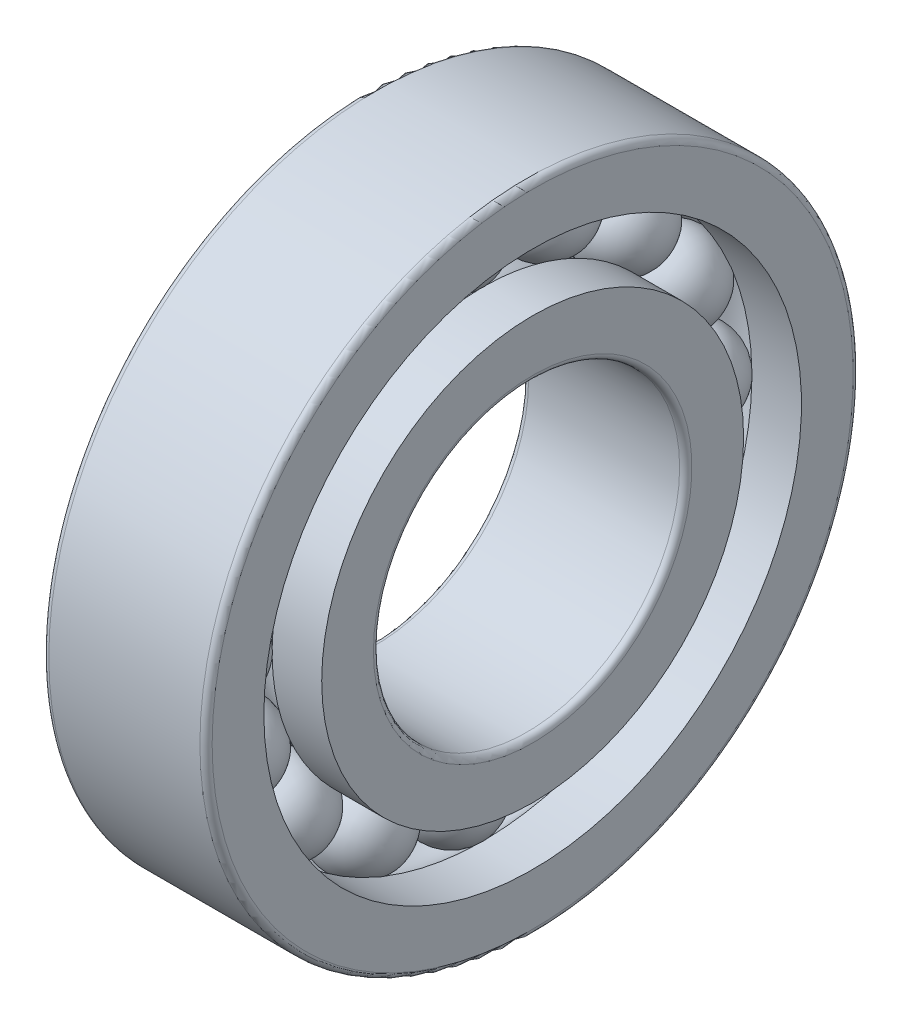
SolidWorks part; units mm, degrees
ref_plane "Front" through (0, 0, 0) normal (0, 0, 1) x (1, 0, 0)
ref_plane "Top" through (0, 0, 0) normal (0, 1, 0) x (1, 0, 0)
ref_plane "Right" through (0, 0, 0) normal (1, 0, 0) x (0, 0, -1)
other "Configuration Table"
sketch "Sketch1" plane through (0, 0, 0) normal (0, 0, 1) x (1, 0, 0)
  line L0 (-9.6833, 0) -> (9.8371, 0) construction
  line L1 (-2.125, 11.75) -> (2.125, 11.75)
  line L2 (-4.5966, 11.75) -> (4.6657, 11.75) construction
  arc A0 (2.125, 11.75) -> (-2.125, 11.75) centre (0, 11.75) ccw
revolve "Revolve1" add sketch "Sketch1" angle 360 about L2
sketch "Sketch2" plane through (0, 0, 0) normal (0, 0, 1) x (1, 0, 0)
  line L0 (-4, 10.3333) -> (-4, 7.5)
  line L1 (-4, 7.5) -> (4, 7.5)
  line L2 (4, 7.5) -> (4, 10.3333)
  line L3 (4, 10.3333) -> (1.5704, 10.3333)
  line L4 (-6.9714, 0) -> (8.1665, 0) construction
  line L5 (-6.7058, 11.75) -> (6.7058, 11.75) construction
  line L6 (-1.5704, 10.3333) -> (-4, 10.3333)
  arc A0 (-1.5704, 10.3333) -> (1.5704, 10.3333) centre (0, 11.75) ccw
revolve "Revolve2" add sketch "Sketch2" angle 360 about L4
sketch "Sketch3" plane through (0, 0, 0) normal (0, 0, 1) x (1, 0, 0)
  line L0 (-8.7107, 0) -> (9.1288, 0) construction
  line L1 (-4, 16) -> (4, 16)
  line L2 (-4, 16) -> (-4, 13.1667)
  line L3 (-4, 13.1667) -> (-1.5704, 13.1667)
  line L4 (4, 16) -> (4, 13.1667)
  line L5 (-7.2948, 11.75) -> (7.2948, 11.75) construction
  line L6 (1.5704, 13.1667) -> (4, 13.1667)
  arc A0 (1.5704, 13.1667) -> (-1.5704, 13.1667) centre (0, 11.75) ccw
revolve "Revolve3" add sketch "Sketch3" angle 360 about L0
pattern_circular "Circular-Pattern1" count 16 over 360 about axis through (0, 0, 0) along (1, 0, 0) of "Revolve1"
fillet "Fillet1" radius 0.3 4 edges at (-4, 0, 7.5) (-4, 0, 16) (4, 0, 16) (4, 0, 7.5)
equation "\"d0@Sketch1\" = ( \"DD@Sketch3\" + \"d@Sketch2\" )  / 2"
equation "\"dia@Sketch1\" =  ( \"DD@Sketch3\" - \"d@Sketch2\" )  / 4"
equation "\"D3@Sketch2\" = ( \"DD@Sketch3\" + \"d@Sketch2\" )  / 2 / 2"
equation "\"D4@Sketch2\" = ( \"DD@Sketch3\" - \"d@Sketch2\" )  / 6"
equation "\"D5@Sketch2\" = \"dia@Sketch1\" - 0.02"
equation "\"B/2@Sketch2\" = \"B@Sketch2\" / 2"
equation "\"D4@Sketch3\" = ( \"DD@Sketch3\" + \"d@Sketch2\" )  / 2 / 2"
equation "\"D5@Sketch3\" = ( \"DD@Sketch3\" - \"d@Sketch2\" )  / 6"
equation "\"B@Sketch3\" = \"B@Sketch2\""
equation "\"B/2@Sketch3\" = \"B@Sketch3\" / 2"
equation "\"D1@Sketch3\" = \"dia@Sketch1\" - 0.02"
equation "\"m@Circular-Pattern1\" = int( 3.14159265 / atn(( \"dia@Sketch1\" / 2) / sqr(( \"DD@Sketch3\" + \"d@Sketch2\" )  / 2 * ( \"DD@Sketch3\" + \"d@Sketch2\" )  / 2/4 - ( \"dia@Sketch1\" / 2) *  ( \"dia@Sketch1\" / 2))))-1"
